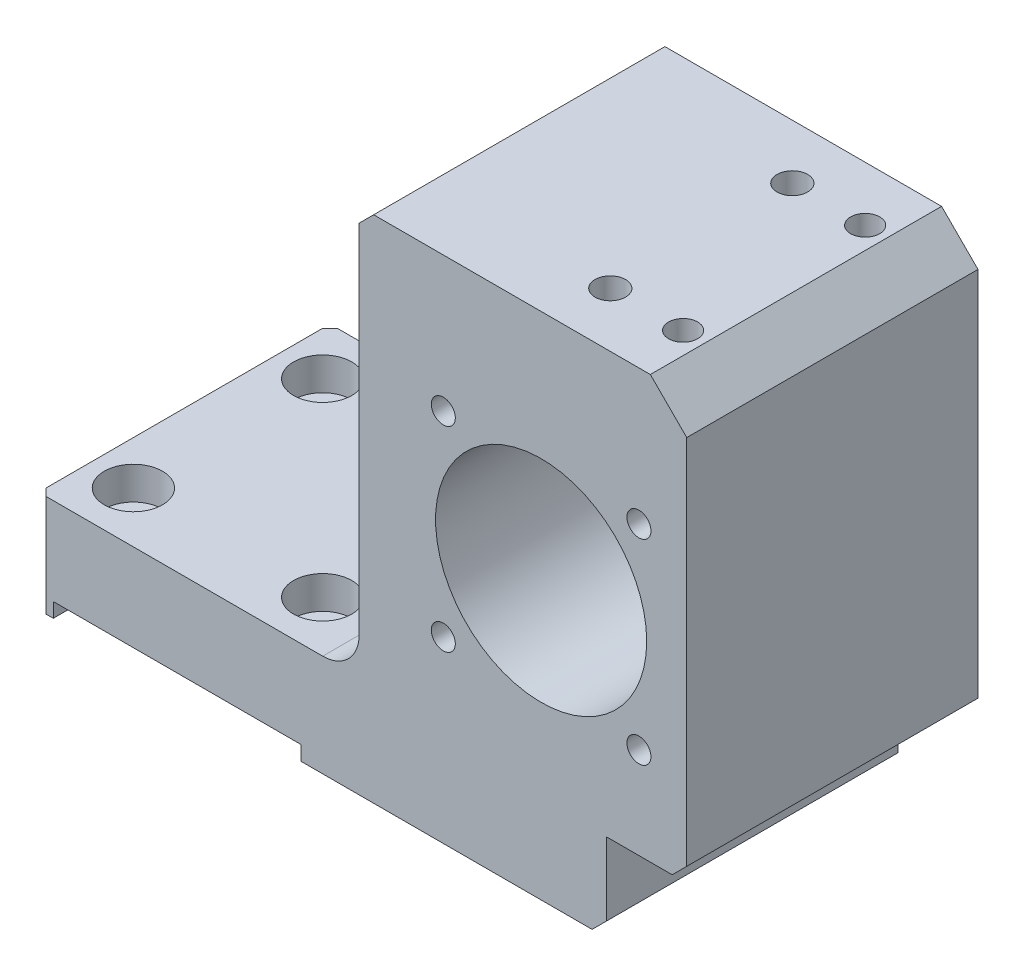
from build123d import *

# Parameters (mm, degrees)
SKETCH1_R                    = 14.5
BOSS_EXTRUDE1_DEPTH          = 20
F_4_5_4_5_DIAMETER_HOLE1_D   = 4.5
SKETCH5_W                    = 34
SKETCH5_H                    = 40
CUT_EXTRUDE1_DEPTH           = 2
M4_TAPPED_HOLE1_D            = 3.3
M4_TAPPED_HOLE1_DEPTH        = 10.1
M4_TAPPED_HOLE1_TIP          = 0.991420021
M5_TAPPED_HOLE1_D            = 4.2
M5_TAPPED_HOLE1_DEPTH        = 14
M5_TAPPED_HOLE1_TIP          = 1.2618073
F_4_0_4_DIAMETER_HOLE1_D     = 4
F_4_0_4_DIAMETER_HOLE1_DEPTH = 12
F_4_0_4_DIAMETER_HOLE1_TIP   = 1.201721238
SKETCH12_W                   = 11
SKETCH12_H                   = 12
CUT_EXTRUDE2_DEPTH           = 121.087468122
M3_TAPPED_HOLE1_D            = 2.5
M3_TAPPED_HOLE1_DEPTH        = 8.5
M3_TAPPED_HOLE1_TIP          = 0.751075774
CHAMFER1_SIZE                = 5
CHAMFER2_SIZE                = 2
SKETCH15_R                   = 4
CUT_EXTRUDE3_DEPTH           = 4.5
FILLET1_R                    = 5
CHAMFER3_SIZE                = 1


with BuildPart() as part:
    # Sketch1 → Boss-Extrude1 (new, symmetric)
    with BuildSketch(Plane.XY):
        Polygon((0, 0), (89, 0), (89, 70), (44, 70), (44, 14), (0, 14), align=None)
        with Locations((69, 38)):
            Circle(SKETCH1_R, mode=Mode.SUBTRACT)
    extrude(amount=BOSS_EXTRUDE1_DEPTH, both=True)

    # Ø4.5 (4.5) Diameter Hole1 (through all)
    with Locations(Plane(origin=(0, 0, 0), x_dir=(-1, 0, 0), z_dir=(0, -1, 0))):
        with Locations((-32, 13), (-6, 13), (-6, -13), (-32, -13)):
            Hole(F_4_5_4_5_DIAMETER_HOLE1_D / 2)

    # Sketch5 → Cut-Extrude1 (cut)
    with BuildSketch(Plane.XZ):
        with Locations((19, 0)):
            Rectangle(SKETCH5_W, SKETCH5_H)
    extrude(amount=-CUT_EXTRUDE1_DEPTH, mode=Mode.SUBTRACT)

    # M4 Tapped Hole1
    with Locations(Plane.XY.offset(20)):
        with Locations((55.564971157, 51.435028843), (82.435028843, 51.435028843), (55.564971157, 24.564971157), (82.435028843, 24.564971157)):
            Hole(M4_TAPPED_HOLE1_D / 2, depth=M4_TAPPED_HOLE1_DEPTH)
            with Locations((0, 0, -(M4_TAPPED_HOLE1_DEPTH + M4_TAPPED_HOLE1_TIP / 2))):  # 118° drill point
                Cone(0, M4_TAPPED_HOLE1_D / 2, M4_TAPPED_HOLE1_TIP, mode=Mode.SUBTRACT)

    # M5 Tapped Hole1
    with Locations(Plane(origin=(0, 70, 0), x_dir=(-1, 0, 0), z_dir=(0, 1, 0))):
        with Locations((-71, -12.5), (-71, 12.5)):
            Hole(M5_TAPPED_HOLE1_D / 2, depth=M5_TAPPED_HOLE1_DEPTH)
            with Locations((0, 0, -(M5_TAPPED_HOLE1_DEPTH + M5_TAPPED_HOLE1_TIP / 2))):  # 118° drill point
                Cone(0, M5_TAPPED_HOLE1_D / 2, M5_TAPPED_HOLE1_TIP, mode=Mode.SUBTRACT)

    # Ø4.0 (4) Diameter Hole1
    with Locations(Plane(origin=(0, 70, 0), x_dir=(-1, 0, 0), z_dir=(0, 1, 0))):
        with Locations((-81, 12.5), (-81, -12.5)):
            Hole(F_4_0_4_DIAMETER_HOLE1_D / 2, depth=F_4_0_4_DIAMETER_HOLE1_DEPTH)
            with Locations((0, 0, -(F_4_0_4_DIAMETER_HOLE1_DEPTH + F_4_0_4_DIAMETER_HOLE1_TIP / 2))):  # 118° drill point
                Cone(0, F_4_0_4_DIAMETER_HOLE1_D / 2, F_4_0_4_DIAMETER_HOLE1_TIP, mode=Mode.SUBTRACT)

    # Sketch12 → Cut-Extrude2 (cut, through all)
    with BuildSketch(Plane.XY.offset(20)):
        with Locations((83.5, 6)):
            Rectangle(SKETCH12_W, SKETCH12_H)
    extrude(amount=-CUT_EXTRUDE2_DEPTH, mode=Mode.SUBTRACT)

    # M3 Tapped Hole1
    with Locations(Plane(origin=(78, 0, 0), x_dir=(0, 0, -1), z_dir=(1, 0, 0))):
        with Locations((-10, 6), (0, 6), (10, 6)):
            Hole(M3_TAPPED_HOLE1_D / 2, depth=M3_TAPPED_HOLE1_DEPTH)
            with Locations((0, 0, -(M3_TAPPED_HOLE1_DEPTH + M3_TAPPED_HOLE1_TIP / 2))):  # 118° drill point
                Cone(0, M3_TAPPED_HOLE1_D / 2, M3_TAPPED_HOLE1_TIP, mode=Mode.SUBTRACT)

    # Chamfer1
    chamfer1_edges = [part.edges().sort_by_distance(p)[0] for p in [
        (89, 70, 0),
    ]]
    chamfer(chamfer1_edges, length=CHAMFER1_SIZE)

    # Chamfer2
    chamfer2_edges = [part.edges().sort_by_distance(p)[0] for p in [
        (44, 70, 0),
        (89, 12, 0),
        (78, 0, 0),
    ]]
    chamfer(chamfer2_edges, length=CHAMFER2_SIZE)

    # Sketch15 → Cut-Extrude3 (cut)
    with BuildSketch(Plane(origin=(0, 14, 0), x_dir=(1, 0, 0), z_dir=(0, 1, 0))):
        with Locations(Location((6, 13, 0), (0, 0, 180))):
            Circle(SKETCH15_R)
        with Locations(Location((32, 13, 0), (0, 0, 180))):
            Circle(SKETCH15_R)
        with Locations(Location((32, -13, 0), (0, 0, 180))):
            Circle(SKETCH15_R)
        with Locations(Location((6, -13, 0), (0, 0, 180))):
            Circle(SKETCH15_R)
    extrude(amount=-CUT_EXTRUDE3_DEPTH, mode=Mode.SUBTRACT)

    # Fillet1
    fillet1_edges = [part.edges().sort_by_distance(p)[0] for p in [
        (44, 14, 0),
    ]]
    fillet(fillet1_edges, radius=FILLET1_R)

    # Chamfer3
    chamfer3_edges = [part.edges().sort_by_distance(p)[0] for p in [
        (0, 7, 20),
        (0, 7, -20),
    ]]
    chamfer(chamfer3_edges, length=CHAMFER3_SIZE)


solid = part.part
